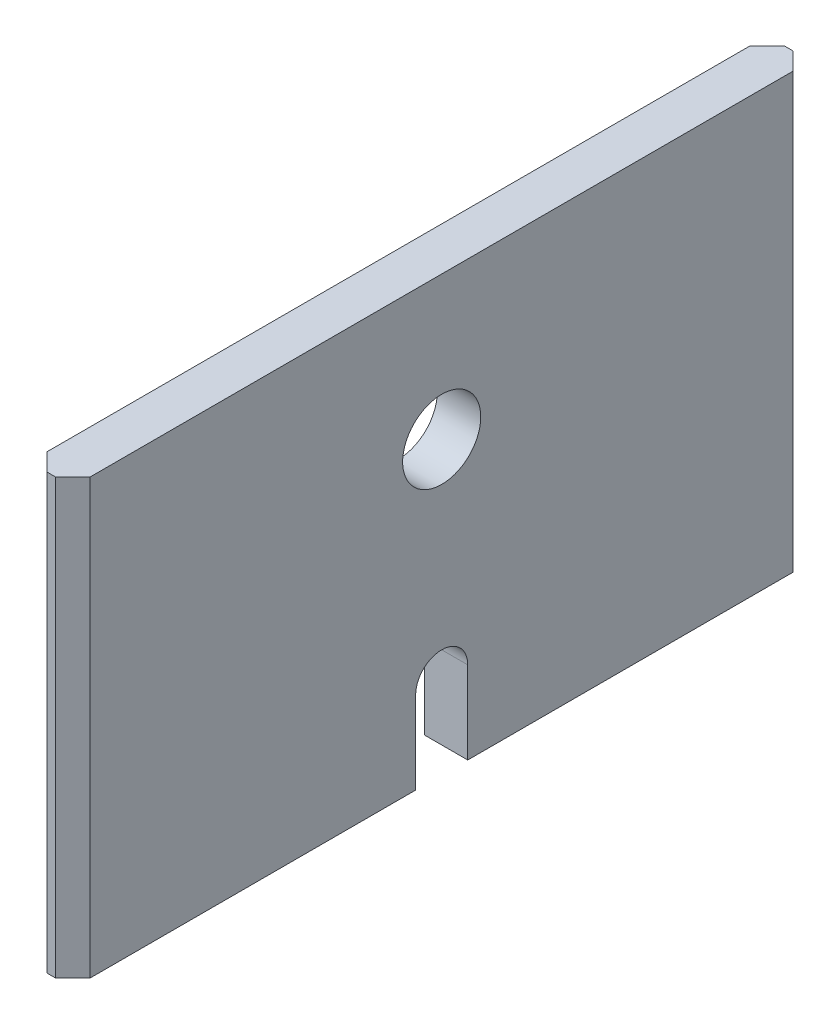
SolidWorks part; units mm, degrees
material "Q235-A"
ref_plane "Front Plane" through (0, 0, 0) normal (0, 0, 1) x (1, 0, 0)
ref_plane "Top Plane" through (0, 0, 0) normal (0, 1, 0) x (1, 0, 0)
ref_plane "Right Plane" through (0, 0, 0) normal (1, 0, 0) x (0, 0, -1)
sketch "Sketch1" plane through (0, 0, 0) normal (1, 0, 0) x (0, 0, -1)
  line L0 (0, -208.1652) -> (0, 208.1652) construction
  line L1 (425, -250) -> (30, -250)
  line L2 (425, -250) -> (425, 250)
  line L3 (425, 250) -> (-425, 250)
  line L4 (-425, -250) -> (-425, 250)
  line L5 (425, -250) -> (-425, 250) construction
  line L6 (425, 250) -> (-425, -250) construction
  line L7 (0, -155) -> (0, -329.2622) construction
  line L8 (30, -155) -> (30, -250)
  line L9 (-30, -155) -> (-30, -250)
  line L10 (-30, -250) -> (-425, -250)
  circle A0 centre (0, 85) radius 45
  arc A1 (30, -155) -> (-30, -155) centre (0, -155) ccw
  point P0 (0, 0)
  point P9 (0, 0)
  point P13 (0, -224.8403)
  dimension "D2" = 500
  dimension "D3" = 90
  dimension "D4" = 335
  dimension "D5" = 30
  dimension "D6" = 95
  dimension "D1" = 850
extrude "Boss-Extrude1" add sketch "Sketch1" along normal mid plane 50
chamfer "Chamfer1" distance 20 angle 45 4 edges at (-25, 0, -425) (25, 0, -425) (-25, 0, 425) (25, 0, 425)
